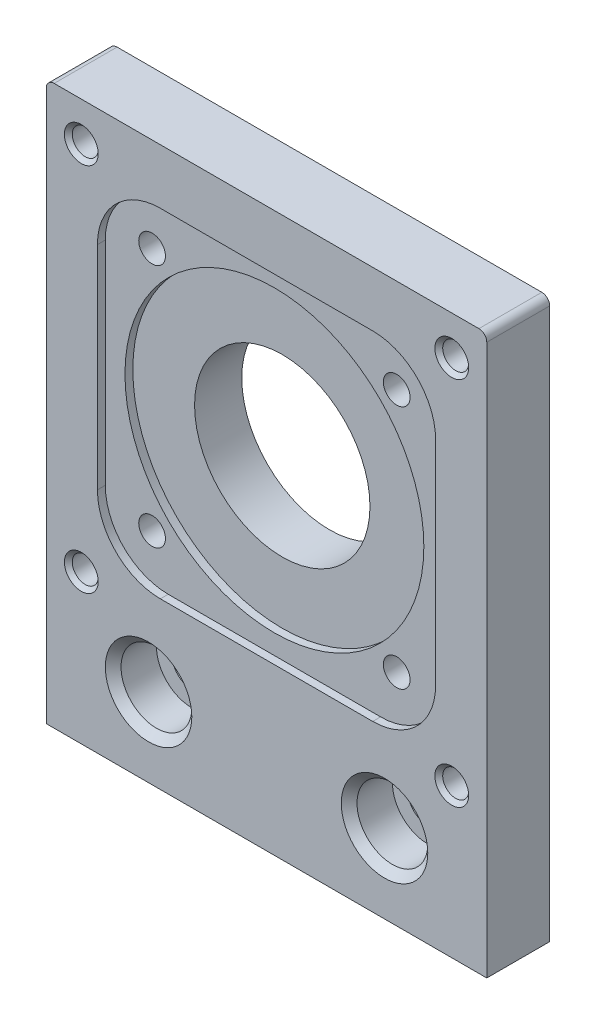
SolidWorks part; units mm, degrees
ref_plane "Front Plane" through (0, 0, 0) normal (0, 0, 1) x (1, 0, 0)
ref_plane "Top Plane" through (0, 0, 0) normal (0, 1, 0) x (1, 0, 0)
ref_plane "Right Plane" through (0, 0, 0) normal (1, 0, 0) x (0, 0, -1)
sketch "Sketch1" plane through (0, 0, 0) normal (0, 0, 1) x (1, 0, 0)
  line L1 (-27, 35.5) -> (27, 35.5)
  line L2 (-28, 34.5) -> (-28, -35.5)
  line L3 (-28, -35.5) -> (28, -35.5)
  line L4 (28, 34.5) -> (28, -35.5)
  line L5 (-28, 35.5) -> (-27.7409, 35.1716) construction
  line L7 (27.7409, 35.1716) -> (28, 35.5) construction
  line L8 (-46.7882, 7) -> (57.1947, 7) construction
  line L10 (0, 35.5) -> (0, -35.5) construction
  line L11 (-44.148, -25.5) -> (59.8348, -25.5) construction
  arc A0 (27, 35.5) -> (28, 34.5) centre (27, 34.5) cw
  arc A1 (-27, 35.5) -> (-28, 34.5) centre (-27, 34.5) ccw
  circle A2 centre (0, 7) radius 11.15
  circle A3 centre (-15.55, 22.55) radius 1.7
  circle A4 centre (-23.55, 30.55) radius 1
  circle A5 centre (23.55, 30.55) radius 1
  circle A6 centre (15.55, 22.55) radius 1.7
  circle A7 centre (-23.55, -16.55) radius 1
  circle A8 centre (-15.55, -8.55) radius 1.7
  circle A9 centre (15.55, -8.55) radius 1.7
  circle A10 centre (23.55, -16.55) radius 1
  circle A11 centre (-15, -25.5) radius 2.5
  circle A12 centre (15, -25.5) radius 2.5
  point P0 (0, 0)
  dimension "D3" = 1
  dimension "D4" = 22.3
  dimension "D6" = 28
  dimension "D8" = 2
  dimension "D9" = 3.4
  dimension "D12" = 5
  dimension "D13" = 5
  dimension "D1" = 56
  dimension "D2" = 71
  dimension "D5" = 42.5
  dimension "D7" = 35.5
  dimension "D10" = 31.1
  dimension "D11" = 47.1
  dimension "D14" = 10
  dimension "D15" = 13
  dimension "D16" = 13
  dimension "D17" = 31.1
  dimension "D18" = 47.1
extrude "Boss-Extrude1" add sketch "Sketch1" along normal blind 8
sketch "Sketch2" plane through (0, 0, 8) normal (0, 0, 1) x (1, 0, 0)
  circle A0 centre (-15, -25.5) radius 4.5
  circle A1 centre (15, -25.5) radius 4.5
  dimension "D1" = 9
  dimension "D2" = 9
extrude "Cut-Extrude1" cut sketch "Sketch2" against normal blind 5.5
sketch "Sketch3" plane through (0, 0, 0) normal (0, 0, -1) x (-1, 0, 0)
  circle A0 centre (-15.55, 22.55) radius 3
  circle A1 centre (15.55, 22.55) radius 3
  circle A2 centre (-15.55, -8.55) radius 3
  circle A3 centre (15.55, -8.55) radius 3
  dimension "D1" = 6
  dimension "D2" = 6
  dimension "D3" = 6
  dimension "D4" = 6
extrude "Cut-Extrude2" cut sketch "Sketch3" against normal blind 4
chamfer "Chamfer1" distance 1 angle 45 4 edges at (12.55, -8.55, 0) (-18.55, -8.55, 0) (-18.55, 22.55, 0) (12.55, 22.55, 0)
chamfer "Chamfer2" distance 0.5 angle 45 4 edges at (24.55, -16.55, 0) (-24.55, -16.55, 0) (-22.55, 30.55, 0) (22.55, 30.55, 0)
chamfer "Chamfer3" distance 0.5 angle 45 4 edges at (-24.55, -16.55, 8) (24.55, -16.55, 8) (22.55, 30.55, 8) (-22.55, 30.55, 8)
sketch "Sketch4" plane through (0, 0, 8) normal (0, 0, 1) x (1, 0, 0)
  circle A0 centre (0, 7) radius 19
  dimension "D1" = 38
extrude "Cut-Extrude3" cut sketch "Sketch4" against normal blind 2
sketch "Sketch5" plane through (0, 0, 8) normal (0, 0, 1) x (1, 0, 0)
  line L1 (-13.5, 28.5) -> (13.5, 28.5)
  line L2 (-21.5, 20.5) -> (-21.5, -6.5)
  line L3 (-13.5, -14.5) -> (13.5, -14.5)
  line L4 (21.5, 20.5) -> (21.5, -6.5)
  line L5 (-21.5, 28.5) -> (21.5, -14.5) construction
  line L6 (-21.5, -14.5) -> (21.5, 28.5) construction
  arc A0 (-21.5, -6.5) -> (-13.5, -14.5) centre (-13.5, -6.5) ccw
  arc A1 (13.5, -14.5) -> (21.5, -6.5) centre (13.5, -6.5) ccw
  arc A2 (13.5, 28.5) -> (21.5, 20.5) centre (13.5, 20.5) cw
  arc A3 (-13.5, 28.5) -> (-21.5, 20.5) centre (-13.5, 20.5) ccw
  point P0 (0, 7)
  dimension "D3" = 8
  dimension "D1" = 43
  dimension "D2" = 43
extrude "Cut-Extrude4" cut sketch "Sketch5" against normal blind 1
chamfer "Chamfer4" distance 1 angle 45 2 edges at (19.5, -25.5, 8) (-10.5, -25.5, 8)
hole_wizard "M4 Tapped Hole1" positions "Sketch9" profile "Sketch8" tap size "M4" standard "Iso" end condition through all
sketch "Sketch9" plane through (0, 0, 8) normal (0, 0, 1) x (1, 0, 0)
  point P0 (-23.55, 30.55)
  point P3 (23.55, 30.55)
  point P6 (23.55, -16.55)
  point P9 (-23.55, -16.55)
sketch "Sketch8" plane through (-23.55, 30.55, 8) normal (1, 0, 0) x (0, -1, 0)
  line L0 (0, 0) -> (0, 8)
  line L1 (0, 8) -> (1.65, 8)
  line L2 (1.65, 8) -> (1.65, 0)
  line L5 (1.65, 0) -> (0, 0)
  line L11 (0, -6.35) -> (0, 107.95) construction
  dimension "通孔螺纹孔钻头直径" = 3.3
  dimension "通孔螺纹孔钻头深度" = 8
cosmetic thread "Cosmetic Thread1" parameters "D2"=4
cosmetic thread "Cosmetic Thread2" parameters "D2"=4
cosmetic thread "Cosmetic Thread3" parameters "D2"=4
cosmetic thread "Cosmetic Thread4" parameters "D2"=4
chamfer "Chamfer5" distance 0.5 angle 45 8 edges at (-21.9, 30.55, 0) (25.2, 30.55, 0) (25.2, -16.55, 0) (-21.9, -16.55, 0) (-21.9, -16.55, 8) (25.2, -16.55, 8) (25.2, 30.55, 8) (-21.9, 30.55, 8)
